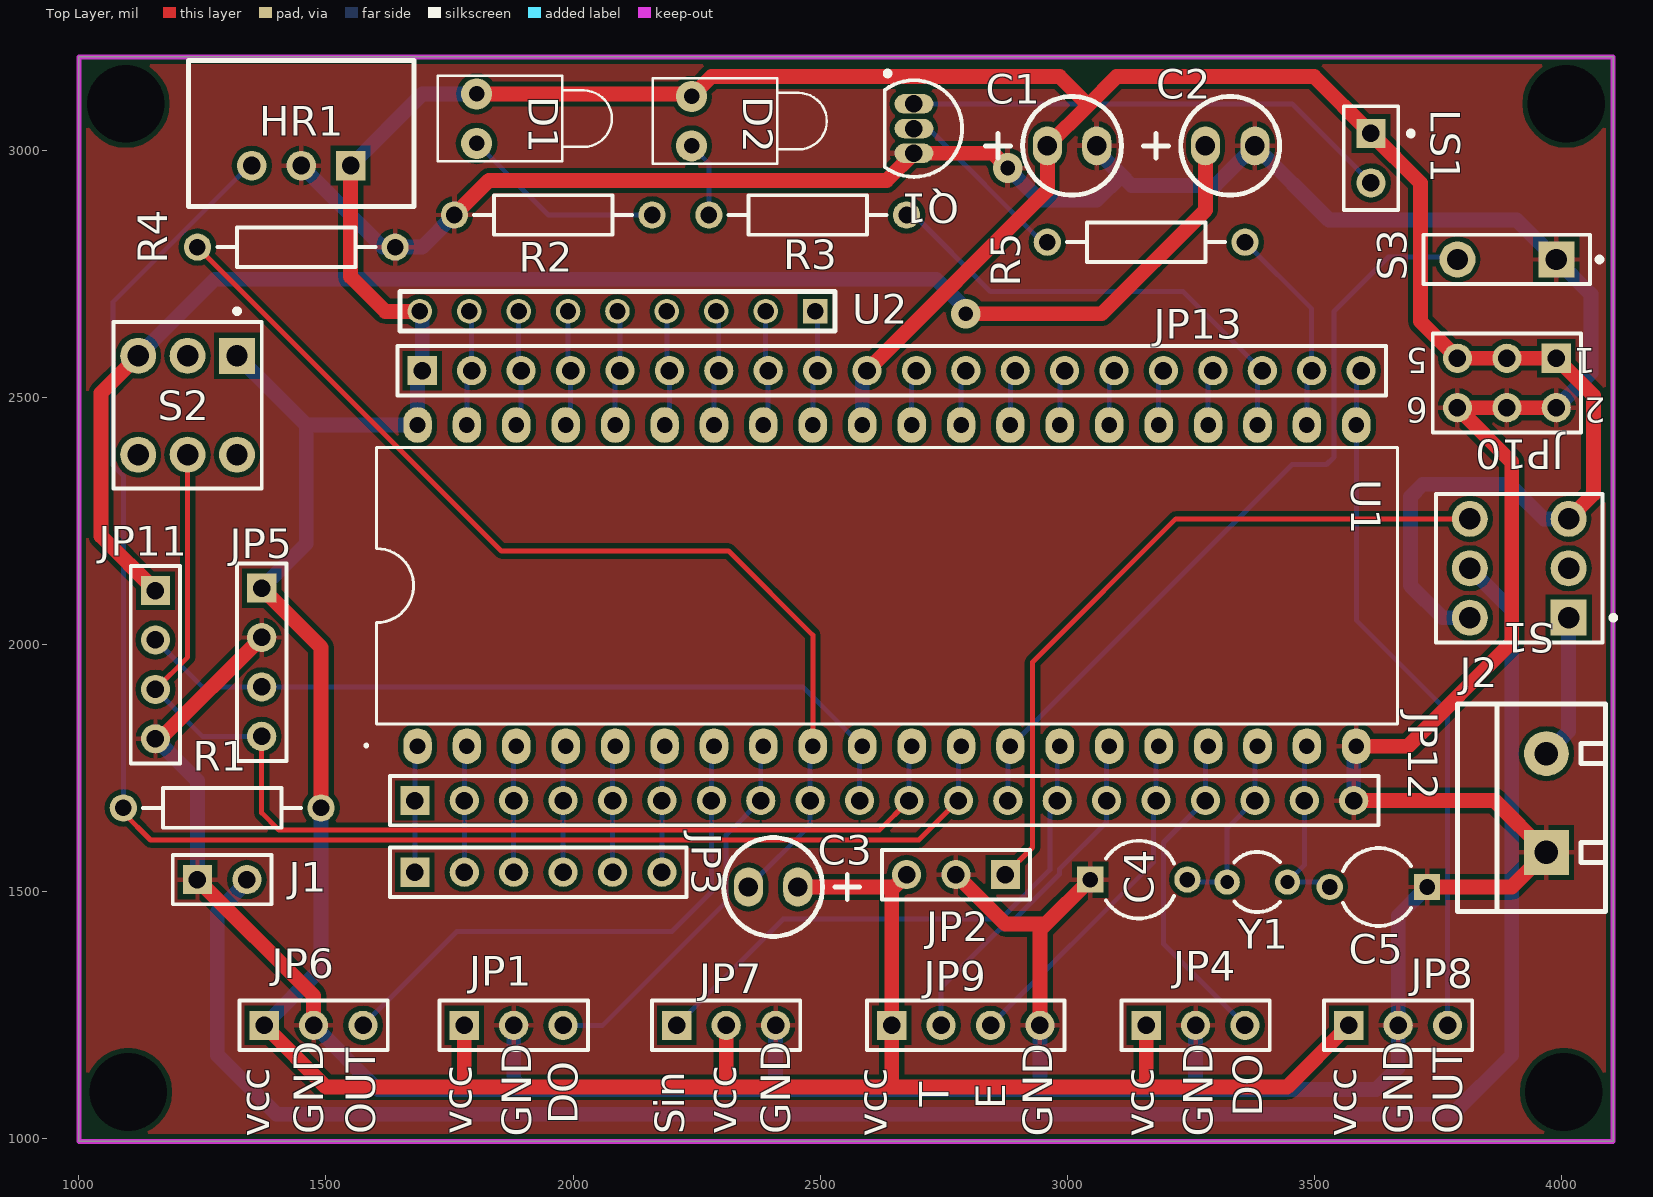
[diagram p0: Top Layer view]
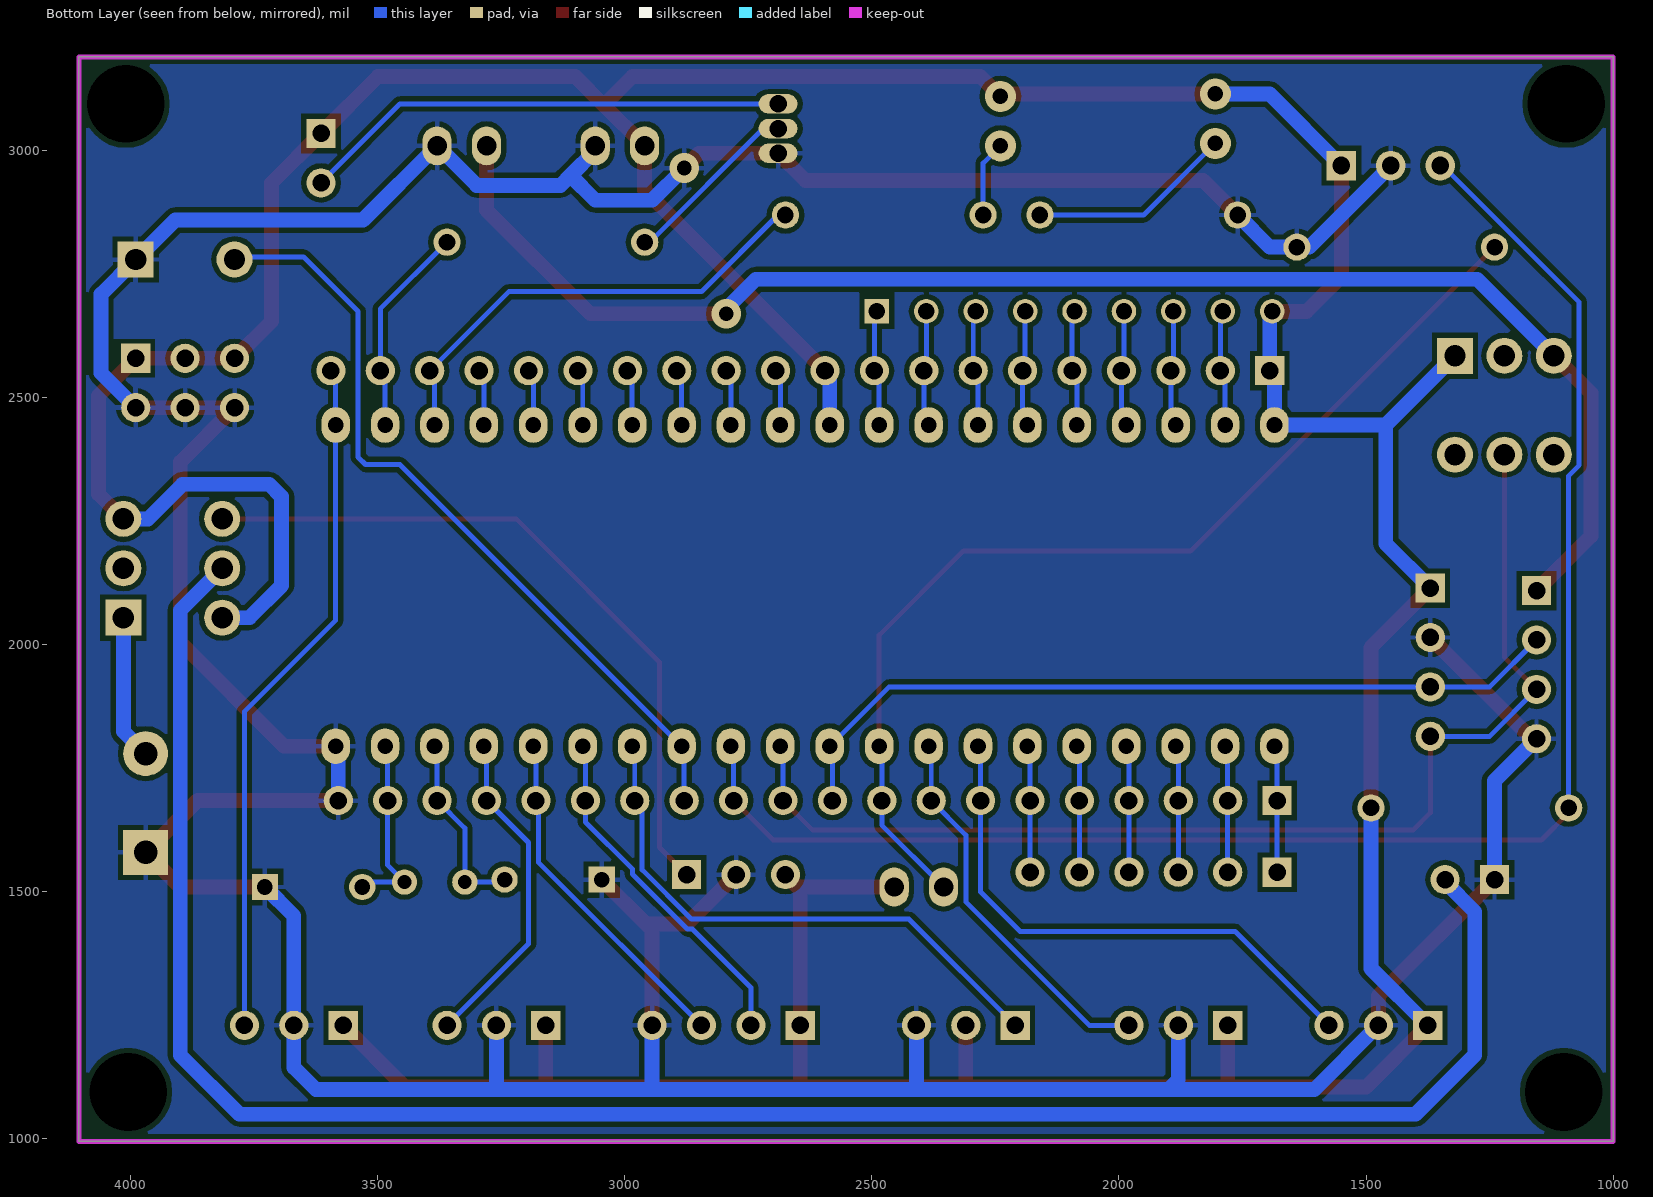
[diagram p1: Bottom Layer view, seen from below]
# Altium PCB MISC82255.PcbDoc
Units mil, origin at the board's own origin, x right, y up, seen from the top; angles counter-clockwise.
Board outline 3105 x 2195 mil, 2 copper layers (Top Layer, Bottom Layer); 36 components, 47 nets, 187 pads, 2 vias.

## Layer stack, top to bottom (the 12.6 mil dielectric is the usual default, probably not edited)
Top Solder: solder mask 0.4, Solder Resist, Dk 3.5
Top Layer: signal copper 1.4
Dielectric 1: dielectric 12.6, FR-4, Dk 4.8
Bottom Layer: signal copper 1.4
Bottom Solder: solder mask 0.4, Solder Resist, Dk 3.5

## Board outline
1000,995 1000,3190 4105,3190 4105,995

## Design rules (kind name [scope] priority, off if disabled: settings)
Clearance [All] p1: gap=10
MinimumSolderMaskSliver [All] p1: minsoldermaskwidth=0
PolygonConnect [All] p1: connectstyle=Relief reliefconductorwidth=10 reliefentries=4 polygonreliefangle="90 Angle" airgapwidth=10
RoutingVias [All] p1: holewidth=28 width=50 viastyle="Through Hole" minholewidth=28 minwidth=50 maxholewidth=28 maxwidth=50
SilkToSilkClearance [All] p1: silktosilkclearance=0
SilkToSolderMaskClearance [IsPad] p1: minsilkscreentomaskgap=0 clearancetoexposedcopper=TRUE
SolderMaskExpansion [All] p1: expansion=4
Width [All] p1: maxlimit=30 minlimit=10 preferedwidth=10
27 further rules are at their usual default settings.

## Components (designator, comment, footprint, x,y, rotation, side; value= is the part's Value field where it differs from the comment)
C1 "470UF" DR 2960,3010 r0 top
C2 "470UF" DR 3280,3010 r0 top
C3 "10UF" DR 2455,1510 r180 top
C4 "22PF" CAPR5-4X5 3145,1525 r0 top
C5 "22PF" CAPR5-4X5 3630,1510 r180 top
D1 "Power" LED-1 1805,3065 r0 top
D2 "Mode indicator LED" LED-1 2240,3060 r0 top
HR1 "HR" SIP3 1450,3035 r180 top
J1 "Header 2" HDR1X2 1240,1525 r0 top
J2 "KF301-2P" KF301-5.0-2P 3970,1580 r90 top
JP1 "Right line tracking" HDR1X3 1780,1230 r0 top
JP2 "L298N power" HDR1X3 2875,1535 r180 top
JP3 "L298N control" HDR1X6 1680,1540 r0 top
JP4 "Left line tracking" HDR1X3 3160,1230 r0 top
JP5 "Bluetooth module" HDR1X4 1370,2115 r270 top
JP6 "Right obstacle avoidance" HDR1X3 1375,1230 r0 top
JP7 "Servo module" HDR1X3 2210,1230 r0 top
JP8 "Left obstacle avoidance" HDR1X3 3570,1230 r0 top
JP9 "Ultrasonic module" HDR1X4 2645,1230 r0 top
JP10 "Header 3X2" HDR2X3 3990,2580 r180 top
JP11 "Download interface" HDR1X4 1155,2110 r270 top
JP12 "Header 20" HDR1X20 1680,1685 r0 top
JP13 "Header 20" HDR1X20 1695,2555 r0 top
LS1 "Bell" PIN2 3615,3035 r270 top
Q1 "2N3906" TO-92A 2690,3045 r180 top
R1 "10K" AXIAL-0.4 1290,1670 r180 top
R2 "1K" AXIAL-0.4 1960,2870 r180 top
R3 "1K" AXIAL-0.4 2475,2870 r0 top
R4 "10K" AXIAL-0.4 1440,2805 r180 top
R5 "1K" AXIAL-0.4 3160,2815 r180 top
S1 "SW-DPDT" DPDT-6 3915,2155 r180 top
S2 "SW-DPDT" DPDT-6 1220,2485 r270 top
S3 "SW-PB" SPST-2 3890,2780 r180 top
U1 "STC89C52RC" STC89C52RC 2625,2120 r0 top
U2 "Resistor network" paizu 2090,2675 r180 top
Y1 "11.05926" R38 3385,1520 r270 top

## Footprints (in the part's own frame and the unit in brackets; to place one, negate y for a bottom-side part, rotate by r counter-clockwise, add the part's x,y. Pads: shape width x height; smd on the part's side, far side on the other; paste and mask are expansions set on the pad)
AXIAL-0.4 [mm] "Axial Device, Thru-Hole; 2 Leads; 0.4 in Pin Spacing"
  round 1.4 hole 0.85: 1(-5.08,0) 2(5.08,0)
  silkscreen extent -4.06,-1.02 4.06,1.02
CAPR5-4X5 [mm] "Capacitor; 2 Leads"
  rect 1.35x1.35 hole 0.8: 1(-2.5,0)
  round 1.35 hole 0.8: 2(2.5,0)
  silkscreen extent -1.69,-2 1.82,2
DPDT-6 [mm] "Switch; 6 Leads"
  rect 1.85x1.85 hole 1.1: 1(-2.54,2.54)
  round 1.85 hole 1.1: 2(-2.54,0) 3(-2.54,-2.54) 4(2.54,-2.54) 5(2.54,0) 6(2.54,2.54)
  silkscreen extent -4.96,-3.81 4.28,3.81
DR [mm]
  oval 1.5x2 hole 1: 1(0,0) 2(2.54,0)
  silkscreen extent -3.17,-2.54 3.81,2.54
HDR1X2 [mm] "Connector; Header; 2 Position"
  rect 1.5x1.5 hole 0.9: 1(0,0)
  round 1.5 hole 0.9: 2(2.54,0)
  silkscreen extent -1.27,-1.27 3.81,1.27
HDR1X3 [mm] "Connector; Header; 3 Position"
  rect 1.5x1.5 hole 0.9: 1(0,0)
  round 1.5 hole 0.9: 2(2.54,0) 3(5.08,0)
  silkscreen extent -1.27,-1.27 6.35,1.27
HDR1X4 [mm] "Connector; Header; 4 Position"
  rect 1.5x1.5 hole 0.9: 1(0,0)
  round 1.5 hole 0.9: 2(2.54,0) 3(5.08,0) 4(7.62,0)
  silkscreen extent -1.27,-1.27 8.89,1.27
HDR1X6 [mm] "Connector; Header; 6 Position"
  rect 1.5x1.5 hole 0.9: 1(0,0)
  round 1.5 hole 0.9: 2(2.54,0) 3(5.08,0) 4(7.62,0) 5(10.16,0) 6(12.7,0)
  silkscreen extent -1.27,-1.27 13.97,1.27
HDR1X20 [mm] "Connector; Header; 20 Position"
  rect 1.5x1.5 hole 0.9: 1(0,0)
  round 1.5 hole 0.9: 2(2.54,0) 3(5.08,0) 4(7.62,0) 5(10.16,0) 6(12.7,0) 7(15.24,0) 8(17.78,0) 9(20.32,0) 10(22.86,0) 11(25.4,0) 12(27.94,0) 13(30.48,0) 14(33.02,0) 15(35.56,0) 16(38.1,0) 17(40.64,0) 18(43.18,0) 19(45.72,0) 20(48.26,0)
  silkscreen extent -1.27,-1.27 49.53,1.27
HDR2X3 [mm] "Connector; Header; 3x2 Position"
  rect 1.5x1.5 hole 0.9: 1(0,0)
  round 1.5 hole 0.9: 2(0,2.54) 3(2.54,0) 4(2.54,2.54) 5(5.08,0) 6(5.08,2.54)
  silkscreen extent -1.27,-1.27 6.35,3.81
KF301-5.0-2P [mm] "可拼接端子/6A"
  rect 2.3x2.3 hole 1.2: 1(0,0)
  round 2.3 hole 1.2: 2(5.08,0)
  silkscreen extent -3.05,-3.05 7.62,4.57, body extent -3,-3.09 7.5,4.51, height 10.05
LED-1 [mm] "LED; 2 Leads"
  round 1.6 hole 0.8: 1(0,1.27) 2(0,-1.27)
  silkscreen extent -2,-2.2 6.95,2.2
paizu [mm]
  rect 1.26x1.26 hole 0.84 paste+0 mask+0.051: 1(-10.16,0)
  round 1.26 hole 0.84 paste+0 mask+0.051: 2(-7.62,0) 3(-5.08,0) 4(-2.54,0) 5(0,0) 6(2.54,0) 7(5.08,0) 8(7.62,0) 9(10.16,0)
  silkscreen extent -11.18,-1.02 11.18,1.02
PIN2 [mm] "Photosensitive Diode; 2 Leads"
  rect 1.5x1.5 hole 0.9: 1(0,0)
  round 1.5 hole 0.9: 2(2.54,0)
  silkscreen extent -1.4,-1.4 3.94,2.18
R38 [mm] "Crystal, Thru-Hole; 2 Leads; Body 3.1 x 8.2 mm (Dia.xH)"
  round 1.3 hole 0.7: 1(0,1.55) 2(0,-1.55)
  silkscreen extent -1.55,-1.19 1.55,1.17
SIP3 [mil]
  rect 60x60 hole 36 paste+0 mask+2: 1(-100,64.96)
  round 60 hole 36 paste+0 mask+2: 2(0,64.96) 3(100,64.96)
  silkscreen extent -228,-148 228,148
SPST-2 [mm] "Switch; 2 Leads"
  rect 1.85x1.85 hole 1.1: 1(-2.54,0)
  round 1.85 hole 1.1: 2(2.54,0)
  silkscreen extent -4.89,-1.27 4.28,1.27
STC89C52RC [mm]
  oval 1.467x1.833 hole 0.8 paste+0 mask+0.051: 1(-23.868,-8.255) 2(-21.328,-8.255) 3(-18.788,-8.255) 4(-16.248,-8.255) 5(-13.708,-8.255) 6(-11.168,-8.255) 7(-8.628,-8.255) 8(-6.088,-8.255) 9(-3.548,-8.255) 10(-1.008,-8.255) 11(1.532,-8.255) 12(4.072,-8.255) 13(6.612,-8.255) 14(9.152,-8.255) 15(11.692,-8.255) 16(14.232,-8.255) 17(16.772,-8.255) 18(19.312,-8.255) 19(21.852,-8.255) 20(24.392,-8.255) 21(24.392,8.255) 22(21.852,8.255) 23(19.312,8.255) 24(16.772,8.255) 25(14.232,8.255) 26(11.692,8.255) 27(9.152,8.255) 28(6.612,8.255) 29(4.072,8.255) 30(1.532,8.255) 31(-1.008,8.255) 32(-3.548,8.255) 33(-6.088,8.255) 34(-8.628,8.255) 35(-11.168,8.255) 36(-13.708,8.255) 37(-16.248,8.255) 38(-18.788,8.255) 39(-21.328,8.255) 40(-23.868,8.255)
  silkscreen extent -26.58,-8.3 26.5,7.11
TO-92A [mm] "TO, Flat Index; 3 In-Line, Axial Leads; Body Dia. 4.5mm; Leads 0.51 x 0.48 mm (max)"
  oval 2x1 hole 0.9: 1(0,-1.27) 2(0,0) 3(0,1.27)
  silkscreen extent -2.48,-2.95 1.5,2.48, body extent -2.48,-2.5 1.5,2.5, height 6.86

## Part data
C1 C2 C3: library part "Cap Pol1", "Polarized Capacitor (Radial)"
C4 C5: library part Cap2, "Capacitor"
D1 D2: library part LED1, "Typical RED GaAs LED"
J1: "Header, 2-Pin"
JP1 JP2 JP4 JP6 JP7 JP8: library part "Header 3", "Header, 3-Pin"
JP3: library part "Header 6", "Header, 6-Pin"
JP5 JP9 JP11: library part "Header 4", "Header, 4-Pin"
JP10: "Header, 3-Pin, Dual row"
JP12 JP13: "Header, 20-Pin"
LS1: "Electrical Bell"
Q1: "PNP General Purpose Amplifier"
R1 R2 R3 R4 R5: library part Res2, "Resistor"
S1 S2: "Double-Pole, Double-Throw Switch"
S3: "Switch"
U2: library part 排阻
Y1: library part XTAL, "Crystal Oscillator"

## Free pads (board coordinates)
  round 118.11 hole 157.48: 0(4010,3095)
  round 78.74 hole 157.48: 1(4005,1095)
  round 39.37 hole 157.48: 2(1100,1095)
  round 59.06 hole 157.48: 3(1095,3095)

## Via types
v1: diameter 60, hole 30, Top Layer to Bottom Layer, 2 vias

## Nets (pads, with @x,y where several pads share a name; then routed paths per layer and width w, separated by ;. In a path a pad name is that pad's centre, name@x,y a point inside that pad or via, vN(x,y) a via of type N, cw(c..) or ccw(c..) an arc to the next point about the centre after c; other vN are vias at no path point)
5V0: C2.1 JP11.1 S2.3 | length 3017.7
  Top Layer w30: S2.3 1045,2510 1045,2220 JP11.1 ; v1(2795,2670) 3070,2670 3280,2880 C2.1
  Bottom Layer w30: S2.3 1275,2740 2735,2740 v1@2795,2680
+5V: J2.2 S1.1 | length 293.6
  Bottom Layer w30: J2.2 4015,1825 S1.1
+12V: J1.2 S1.5 | length 4119.5
  Bottom Layer w30: J1.2 1340,1520 1280,1460 1280,1170 1400,1050 3780,1050 3899.72,1169.72 3899.72,1809.11 3900,1809.38 3900,2070 S1.5
ALE: JP13.11 U1.30 | length 114
  Bottom Layer w10: U1.30 2685.33,2545.33 JP13.11
GND: C1.2 C2.2 C4.1 C5.1 HR1.2 J1.1 J2.1 JP1.2 JP2.2 JP4.2 JP5.2 JP6.2 JP7.3 JP8.2 JP9.4 JP10.2 JP10.4 JP10.6 JP11.4 JP12.20 Q1.3 R2.2 R4.1 S3.1 U1.20 | length 10024.7
  Top Layer w30: JP11.4 1165,1810 JP5.2 ; J1.1 1475,1290 JP6.2 ; R2.2 1830,2940 2635,2940 Q1.3 2850,2995 v1(2880,2965) ; JP2.2 2875,1435 2956.57,1435 ; JP9.4 2945,1423.43 2956.57,1435 ; C4.1 2956.57,1435 ; JP12.20 3865,1685 J2.1 3900,1510 C5.1 ; U1.20 3690,1795 3900,2005 3900,2370 JP10.6 JP10.4 JP10.2
  Bottom Layer w10: U1.20@3580,1789.67 U1.20
  Bottom Layer w30: JP11.4 1240,1725 J1.1 ; HR1.2 1615.04,2805 R4.1 1695,2805 R2.2 ; JP6.2 1605,1100 1900,1100 ; JP1.2 1880,1120 1900,1100 ; JP7.3 2410,1105 2415,1100 ; v1(2880,2965) 2945,2900 3060,2900 3110,2950 ; JP9.4 2945,1105 2940,1100 ; C1.2 3060,3000 3110,2950 ; JP4.2 3260,1105 3255,1100 ; JP12.20 U1.20@3580,1789.67 ; C5.1 3670,1451.57 JP8.2 3670,1145 3625,1100 3255,1100 ; JP10.2 4060,2550 4060,2710 S3.1 3910,2860 3530,2860 C2.2 3300,2930 3130,2930 3110,2950 ; 1900,1100 2415,1100 ; 2415,1100 2940,1100 ; 2940,1100 3255,1100
NetD1_2: D1.2 R2.1 | length 415.1
  Bottom Layer w10: D1.2 1950,2870 R2.1
NetD2_2: D2.2 R3.1 | length 154.5
  Bottom Layer w10: D2.2 2275,2975 R3.1
NetJP2_1: JP2.1 S1.4 | length 1457.9
  Top Layer w10: JP2.1 2930,1590 2930,1965 3220,2255 S1.4
NetLS1_2: LS1.2 Q1.1 | length 991.3
  Bottom Layer w10: Q1.1 3455,3095 LS1.2
NetQ1_2: Q1.2 R5.2 | length 365.3
  Bottom Layer w10: Q1.2 2720,3045 2950,2815 R5.2
P00: JP13.2 U1.39 U2.8 | length 236.1
  Bottom Layer w10: U1.39 1785.33,2545.33 JP13.2 1795,2670 U2.8
P01: JP13.3 U1.38 U2.7 | length 236.1
  Bottom Layer w10: U1.38 1895,2454.67 JP13.3 1890,2560 U2.7
P02: JP13.4 U1.37 U2.6 | length 236.1
  Bottom Layer w10: U1.37 1995,2454.67 JP13.4 1990,2560 U2.6
P03: JP13.5 U1.36 U2.5 | length 236.1
  Bottom Layer w10: U1.36 2085.33,2545.33 JP13.5 2095,2670 U2.5
P04: JP13.6 U1.35 U2.4 | length 236.1
  Bottom Layer w10: U1.35 2195,2454.67 JP13.6 2190,2560 U2.4
P05: JP13.7 U1.34 U2.3 | length 236.1
  Bottom Layer w10: U1.34 2285.33,2545.33 JP13.7 2295,2670 U2.3
P06: JP13.8 U1.33 U2.2 | length 236.1
  Bottom Layer w10: U1.33 2395,2454.67 JP13.8 2390,2560 U2.2
P07: JP13.9 U1.32 U2.1 | length 236.1
  Bottom Layer w10: U1.32 2485.33,2545.33 JP13.9 2495,2670 U2.1
P10: JP3.1 JP12.1 U1.1 | length 257.2
  Bottom Layer w10: JP3.1 JP12.1 1680,1789.67 U1.1
P11: JP3.2 JP12.2 U1.2 | length 257.2
  Bottom Layer w10: JP3.2 JP12.2 1780,1789.67 U1.2
P12: JP3.3 JP12.3 U1.3 | length 257.2
  Bottom Layer w10: JP3.3 JP12.3 1880,1789.67 U1.3
P13: JP3.4 JP12.4 U1.4 | length 257.2
  Bottom Layer w10: JP3.4 JP12.4 1980,1789.67 U1.4
P14: JP3.5 JP12.5 U1.5 | length 257.2
  Bottom Layer w10: JP3.5 JP12.5 2080,1789.67 U1.5
P15: JP3.6 JP12.6 U1.6 | length 257.2
  Bottom Layer w10: JP3.6 JP12.6 2180,1789.67 U1.6
P16: JP6.3 JP12.7 U1.7 | length 1114
  Bottom Layer w10: JP6.3 1765,1420 2200,1420 2280,1500 JP12.7 2280,1789.67 U1.7
P17: JP1.3 JP12.8 U1.8 | length 779.8
  Bottom Layer w10: JP1.3 2060,1230 2310,1480 2310,1615 JP12.8 2380,1789.67 U1.8
P20: JP8.3 JP13.20 U1.21 | length 1405.5
  Bottom Layer w10: JP13.20 3585.33,2545.33 U1.21 3585.33,2049.67 3770,1865 JP8.3
P21: JP13.19 R5.1 U1.22 | length 429.9
  Bottom Layer w10: R5.1 3495,2680 JP13.19 3485.33,2545.33 U1.22
P22: JP13.18 R3.2 U1.23 | length 964.5
  Bottom Layer w10: R3.2 2690,2870 2845,2715 3235,2715 JP13.18 3385.33,2545.33 U1.23
P23: JP13.17 U1.24 | length 114
  Bottom Layer w10: U1.24 3285.33,2545.33 JP13.17
P24: JP13.16 U1.25 | length 114
  Bottom Layer w10: U1.25 3185.33,2545.33 JP13.16
P25: JP13.15 U1.26 | length 114
  Bottom Layer w10: U1.26 3085.33,2545.33 JP13.15
P26: JP13.14 U1.27 | length 114
  Bottom Layer w10: U1.27 2985.33,2545.33 JP13.14
P27: JP13.13 U1.28 | length 114
  Bottom Layer w10: U1.28 2885.33,2545.33 JP13.13
P30: JP5.3 JP11.2 JP12.10 U1.10 | length 1631.6
  Bottom Layer w10: JP11.2 1250,1915 JP5.3 2465.33,1915 U1.10 2580,1789.67 JP12.10
P31: JP5.4 JP11.3 JP12.11 S2.5 U1.11 | length 2372.8
  Top Layer w10: JP11.3 1220,1975 S2.5 ; JP5.4 1370,1660 1405,1625 2620,1625 JP12.11
  Bottom Layer w10: JP11.3 1250,1815 JP5.4 ; JP12.11 2680,1789.67 U1.11
P32: HR1.3 JP12.12 R1.2 U1.12 | length 3296.6
  Top Layer w10: R1.2@1090,1660 1145,1605 2700,1605 JP12.12
  Bottom Layer w10: R1.2@1090,1660 R1.2 1090,2342.28 1068.58,2363.7 1068.58,2693.77 1344.85,2970.04 HR1.3 ; JP12.12 2780,1789.67 U1.12
P33: JP12.13 S3.2 U1.13 | length 1601.8
  Bottom Layer w10: JP12.13 2880,1789.67 U1.13 3455.33,2365 3525,2365 3540,2380 3540,2675 3650,2785 3785,2785 S3.2
P34: JP7.1 JP12.14 U1.14 | length 1144.1
  Bottom Layer w10: JP7.1 2425,1445 2865.27,1445 2965,1544.73 2965,1670 JP12.14 2980,1789.67 U1.14
P35: JP9.2 JP12.15 U1.15 | length 711.9
  Bottom Layer w10: JP9.2 2745,1306.58 2863.43,1425 2873.55,1425 2985,1536.45 2985,1546.58 3080,1641.58 JP12.15 3080,1789.67 U1.15
P36: JP9.3 JP12.16 U1.16 | length 706
  Bottom Layer w10: JP9.3 3175,1560 3175,1680 JP12.16 3180,1789.67 U1.16
P37: JP4.3 JP12.17 U1.17 | length 670.8
  Bottom Layer w10: U1.17 3280,1789.67 JP12.17 3195,1600 3195,1395 JP4.3
PSEN: JP13.12 U1.29 | length 114
  Bottom Layer w10: U1.29 2785.33,2545.33 JP13.12
RST: C3.2 JP12.9 R4.2 U1.9 | length 2134.3
  Top Layer w10: R4.2 1855,2190 2315,2190 2485.33,2019.67 U1.9
  Bottom Layer w10: C3.2 2480,1635 JP12.9 2480,1789.67 U1.9
VCC: C1.1 C3.1 D1.1 D2.1 HR1.1 JP1.1 JP2.3 JP4.1 JP5.1 JP6.1 JP7.2 JP8.1 JP9.1 JP10.1 JP10.3 JP10.5 JP13.1 JP13.10 LS1.1 R1.1 S1.3 S1.6 S2.1 U1.31 U1.40 U2.9 | length 10590.7
  Top Layer w30: JP5.1 1490,1995 R1.1 R1.1@1490,1660 ; JP6.1 1500,1105 1775,1105 ; HR1.1 1550,2745 1620,2675 U2.9 ; JP1.1 1780,1110 1775,1105 ; D1.1 2235,3115 D2.1 2280,3150 2985,3150 3042.5,3092.5 ; JP7.2 2310,1110 2305,1105 ; C3.1 2650,1510 ; JP13.10 2960,2920 C1.1 3042.5,3092.5 ; JP2.3 2650,1510 ; JP4.1 3160,1115 3150,1105 ; JP8.1 3445,1105 3150,1105 ; S1.3 4065,2305 4065,2505 JP10.1 JP10.3 JP10.5 3715,2655 3715,2935 LS1.1 3500,3150 3100,3150 3042.5,3092.5 ; 1775,1105 2305,1105 ; 2305,1105 2650,1105 ; 2650,1105 3150,1105 ; 2650,1105 2645,1110 JP9.1 2645,1505 2650,1510
  Bottom Layer w30: S2.1 1460,2445 ; JP5.1 1460,2205 1460,2445 ; JP6.1 1490,1345 R1.1@1490,1660 ; HR1.1 1694.96,3115 D1.1 ; U2.9 1695,2670 JP13.1 1685.33,2545.33 U1.40 1460,2445 ; U1.31 2585.33,2545.33 JP13.10 ; S1.6 3760,2055 3695,2120 3695,2300 3720,2325 3895,2325 3965,2255 S1.3
X1: C5.2 JP12.19 U1.19 Y1.1 | length 381
  Bottom Layer w10: U1.19 3480,1789.67 JP12.19 3480,1553.98 Y1.1 3521.57,1520 C5.2
X2: C4.2 JP12.18 U1.18 Y1.2 | length 383
  Bottom Layer w10: C4.2 3248.43,1520 Y1.2 3323.98,1628.98 JP12.18 3380,1789.67 U1.18
pads on no net: S1.2 S2.2 S2.4 S2.6

## Polygon pours and split planes (outlines as drawn)
GND on Bottom Layer "Top Layer-No Net" (solid, remove dead copper, pour order 0): 660,3515 790,3385 4280,3385 4280,650 4350,580 4270,660 875,660
GND on Top Layer "Top Layer-No Net" (solid, remove dead copper, pour order 2): 580,3430 4400,3430 4450,3480 4460,3470 4460,460 1340,460 1080,720 1020,780 930,780

## Keep-outs
Keep-Out Layer:
  the board outline again, w10

## Silkscreen, mask and mechanical layers (free items; w line width, h text height)
Top Overlay:
  text "T" at 2760,1065 h60 r90
  text "E" at 2875,1060 h60 r90
  text "DO" at 3395,1045 h60 r90
  text "DO" at 2010,1030 h60 r90
  text "GND" at 1495,1010 h60 r90
  text "OUT" at 1600,1010 h60 r90
  text "vcc" at 1795,1010 h60 r90
  text "Sin" at 2225,1010 h60 r90
  text "vcc" at 2330,1010 h60 r90
  text "GND" at 2440,1010 h60 r90
  text "GND" at 3700,1010 h60 r90
  text "OUT" at 3800,1010 h60 r90
  text "vcc" at 1385,1005 h60 r90
  text "GND" at 1915,1005 h60 r90
  text "vcc" at 2635,1005 h60 r90
  text "GND" at 2970,1005 h60 r90
  text "vcc" at 3175,1005 h60 r90
  text "GND" at 3295,1005 h60 r90
  text "vcc" at 3585,1005 h60 r90